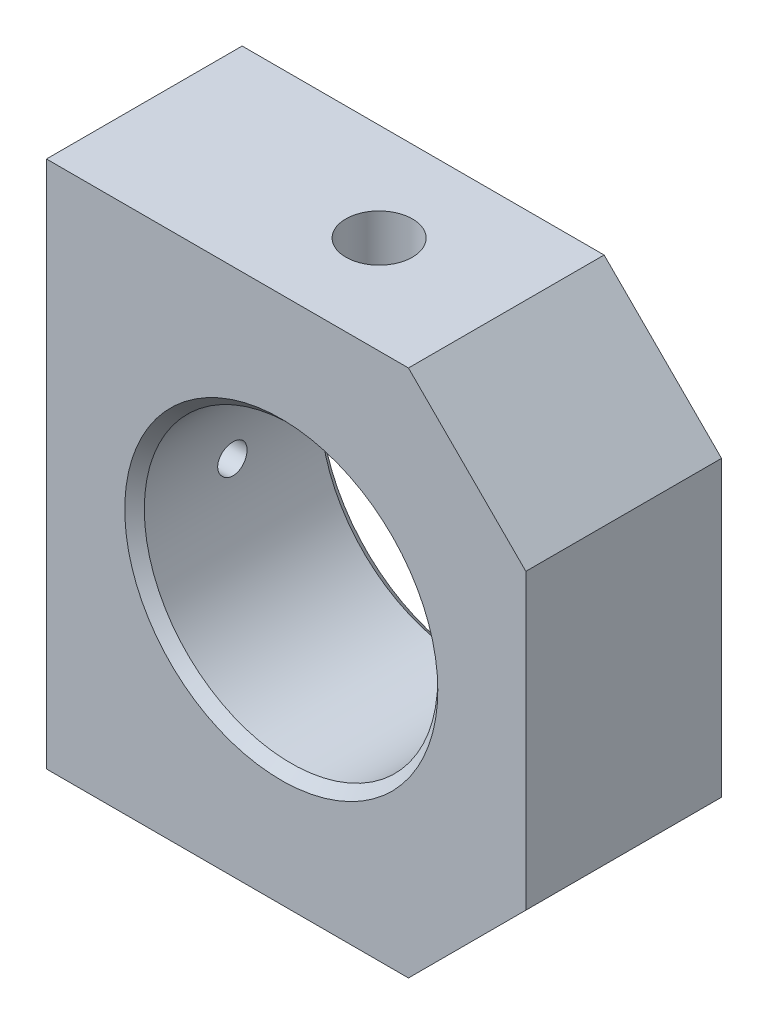
SolidWorks part; units mm, degrees
material "1023 碳钢板 (SS)"
ref_plane "Front Plane" through (0, 0, 0) normal (0, 0, 1) x (1, 0, 0)
ref_plane "Top Plane" through (0, 0, 0) normal (0, 1, 0) x (1, 0, 0)
ref_plane "Right Plane" through (0, 0, 0) normal (1, 0, 0) x (0, 0, -1)
sketch "Sketch1" plane through (0, 0, 0) normal (0, 0, 1) x (1, 0, 0)
  line L0 (12.5, 27) -> (24.5, 15)
  line L1 (-24.5, 27) -> (12.5, 27)
  line L2 (-24.5, 27) -> (-24.5, -27)
  line L3 (-24.5, -27) -> (12.5, -27)
  line L4 (24.5, 15) -> (24.5, -15)
  line L5 (-24.5, 27) -> (24.5, -27) construction
  line L6 (-24.5, -27) -> (24.5, 27) construction
  line L7 (12.5, -27) -> (24.5, -15)
  point P0 (0, 0)
  dimension "D1" = 49
  dimension "D2" = 54
  dimension "D3" = 12
  dimension "D4" = 45
  dimension "D5" = 12
  dimension "D6" = 45
extrude "Boss-Extrude1" add sketch "Sketch1" along normal blind 20
sketch "Sketch2" plane through (0, 0, 20) normal (0, 0, 1) x (1, 0, 0)
  line L0 (-24.5, 27) -> (-24.5, -27) construction
  circle A2 centre (-0.5, 0) radius 15
  dimension "D1" = 24
  dimension "D2" = 30
extrude "Cut-Extrude1" cut sketch "Sketch2" against normal blind 20
hole_wizard "M8 Tapped Hole1" positions "3DSketch1" profile "Sketch3" tap size "M8" standard "IS"
sketch3d "3DSketch1"
  line L0 (-24.5, 27, 20) -> (-24.5, 27, 0) construction
  line L1 (12.5, 27, 0) -> (-24.5, 27, 0) construction
  point P0 (-0.5, 27, 10)
  dimension "D1" = 24
  dimension "D2" = 10
sketch "Sketch3" plane through (-0.5, 27, 10) normal (1, 0, 0) x (0, 0, 1)
  line L0 (0, 0) -> (0, 17.0429)
  line L1 (0, 17.0429) -> (3.4, 15)
  line L2 (3.4, 15) -> (3.4, 0)
  line L5 (3.4, 0) -> (0, 0)
  line L10 (0, 17.0429) -> (-3.4, 15) construction
  line L11 (0, -6.35) -> (0, 107.95) construction
  dimension "螺纹孔钻头直径" = 6.8
  dimension "螺纹孔钻头深度" = 15
  dimension "导头角度" = 118
cosmetic thread "Hole thread 1" parameters "D1"=16, "D2"=8
chamfer "Chamfer2" distance 1 angle 45 2 edges at (14.5, 0, 0) (14.5, 0, 20)
hole_wizard "Size mm dowel hole 1" positions "3DSketch2" profile "Sketch4" hole size "Ø3.0" standard "IS"
sketch3d "3DSketch2"
  line L0 (-24.5, 27, 0) -> (-24.5, -27, 0) construction
  line L1 (-24.5, 27, 20) -> (-24.5, 27, 0) construction
  point P0 (-24.5, 0, 10)
  dimension "D1" = 10
  dimension "D2" = 27
sketch "Sketch4" plane through (-24.5, 0, 10) normal (0, 1, 0) x (0, 0, 1)
  line L0 (0, 0) -> (0, 20.6513)
  line L1 (0, 20.6513) -> (1.5, 19.75)
  line L2 (1.5, 19.75) -> (1.5, 0)
  line L5 (1.5, 0) -> (0, 0)
  line L10 (0, 20.6513) -> (-1.5, 19.75) construction
  line L11 (0, -6.35) -> (0, 107.95) construction
  dimension "孔直径" = 3
  dimension "孔深度" = 19.75
  dimension "导头角度" = 118
